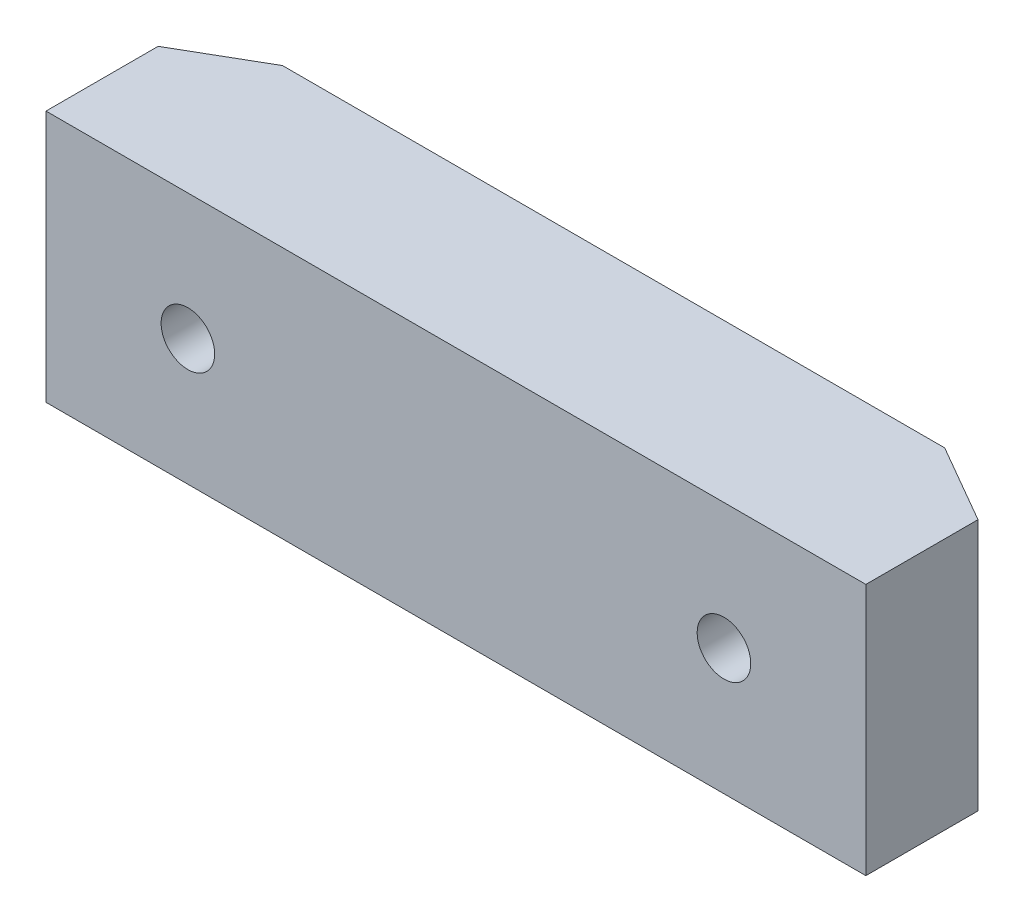
SolidWorks part; units mm, degrees
material "商用纯等级 2 纵向 (SS)"
ref_plane "前视基准面" through (0, 0, 0) normal (0, 0, 1) x (1, 0, 0)
ref_plane "上视基准面" through (0, 0, 0) normal (0, 1, 0) x (1, 0, 0)
ref_plane "右视基准面" through (0, 0, 0) normal (1, 0, 0) x (0, 0, -1)
sketch "草图1" plane through (0, 0, 0) normal (0, 0, 1) x (1, 0, 0)
  line L1 (26, -8) -> (-26, -8)
  line L2 (26, -8) -> (26, 8)
  line L3 (26, 8) -> (-26, 8)
  line L4 (-26, -8) -> (-26, 8)
  line L5 (26, -8) -> (-26, 8) construction
  line L6 (26, 8) -> (-26, -8) construction
  point P0 (0, 0)
  dimension "D1" = 52
  dimension "D2" = 16
extrude "凸台-拉伸1" add sketch "草图1" along normal blind 10
hole_wizard "打孔尺寸(%根据)内六角圆柱头螺钉的类型1" positions "草图2" profile "草图3" counterbore size "M3" standard "GB"
sketch "草图2" plane through (0, 0, 0) normal (0, 0, -1) x (-1, 0, 0)
  point P0 (-17, 0)
  point P4 (17, 0)
sketch "草图3" plane through (17, 0, 0) normal (1, 0, 0) x (0, 1, 0)
  line L0 (0, 0) -> (0, 39.0215)
  line L1 (0, 39.0215) -> (1.7, 38)
  line L2 (1.7, 38) -> (1.7, 3.4)
  line L3 (1.7, 3.4) -> (3, 3.4)
  line L4 (3, 3.4) -> (3, 0)
  line L5 (3, 0) -> (0, 0)
  line L10 (0, 39.0215) -> (-1.7, 38) construction
  line L11 (0, -6.35) -> (0, 107.95) construction
  dimension "孔直径" = 3.4
  dimension "孔深度" = 38
  dimension "柱形沉头孔直径" = 6
  dimension "柱形沉头孔深度" = 3.4
  dimension "导头角度" = 118
chamfer "倒角1" distance 5 angle 30 1 edges at (26, 0, 0)
chamfer "倒角2" distance 5 angle 30 1 edges at (-26, 0, 0)
